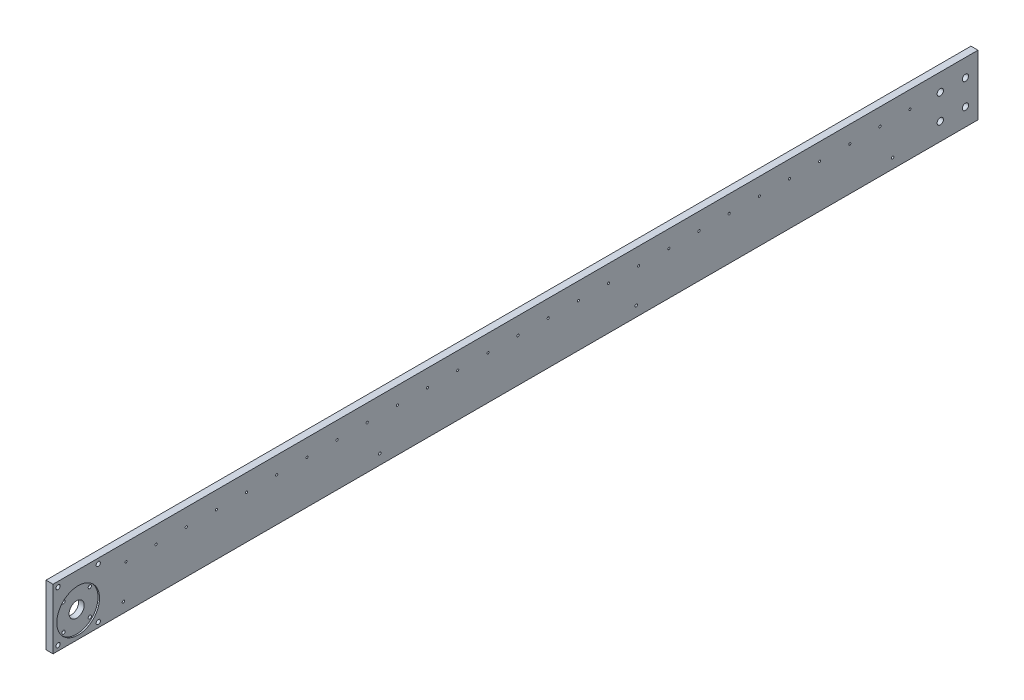
SolidWorks part; units mm, degrees
ref_plane "前视基准面" through (0, 0, 0) normal (0, 0, 1) x (1, 0, 0)
ref_plane "上视基准面" through (0, 0, 0) normal (0, 1, 0) x (1, 0, 0)
ref_plane "右视基准面" through (0, 0, 0) normal (1, 0, 0) x (0, 0, -1)
sketch "草图1" plane through (0, 0, 0) normal (1, 0, 0) x (0, 0, -1)
  line L1 (-920, 60) -> (920, 60)
  line L2 (-920, 60) -> (-920, -60)
  line L3 (-920, -60) -> (920, -60)
  line L4 (920, 60) -> (920, -60)
  line L5 (-920, 60) -> (920, -60) construction
  line L6 (-920, -60) -> (920, 60) construction
  point P0 (0, 0)
  dimension "D1" = 1840
  dimension "D2" = 120
extrude "凸台-拉伸1" add sketch "草图1" along normal blind 14
hole_wizard "打孔尺寸(%根据)内六角圆柱头螺钉的类型1" positions "草图2" profile "草图3" counterbore size "M6" standard "GB" end condition through all
sketch "草图2" plane through (0, 0, 0) normal (1, 0, 0) x (0, 0, -1)
  line L0 (-860, -10) -> (-727.1684, -10) construction
  line L4 (920, 60) -> (-920, 60) construction
  line L5 (-843.837, 16.163) -> (-896.163, 16.163) construction
  line L7 (-843.837, 16.163) -> (-843.837, -36.163) construction
  line L9 (-870, 16.163) -> (-870, -28.2194) construction
  line L11 (-843.837, -10) -> (-896.4633, -10) construction
  line L13 (-843.837, 16.163) -> (-870, -10) construction
  line L14 (-920, 60) -> (-920, -60) construction
  point P0 (-896.163, 16.163)
  point P2 (-843.837, 16.163)
  point P4 (-896.163, -36.163)
  point P6 (-843.837, -36.163)
  dimension "D2" = 45
  dimension "D1" = 70
  dimension "D3" = 37
  dimension "D4" = 50
sketch "草图3" plane through (0, 16.163, 896.163) normal (0, 1, 0) x (0, 0, 1)
  line L0 (0, 0) -> (0, 14)
  line L1 (0, 14) -> (3.3, 14)
  line L3 (3.3, 14) -> (3.3, 6.8)
  line L4 (3.3, 6.8) -> (5.5, 6.8)
  line L5 (5.5, 6.8) -> (5.5, 0)
  line L7 (5.5, 0) -> (0, 0)
  line L11 (0, -6.35) -> (0, 107.95) construction
  dimension "通孔孔直径" = 6.6
  dimension "通孔孔深度" = 14
  dimension "柱形沉头孔直径" = 11
  dimension "柱形沉头孔深度" = 6.8
hole_wizard "M5 螺纹孔1" positions "草图4" profile "草图5" tap size "M5" standard "GB" end condition through all
sketch "草图4" plane through (14, 0, 0) normal (1, 0, 0) x (0, 0, -1)
  line L0 (-920, 60) -> (-920, -60) construction
  line L1 (-920, -60) -> (920, -60) construction
  point P0 (-775, 26)
  dimension "D1" = 145
  dimension "D2" = 86
sketch "草图5" plane through (14, 26, 775) normal (0, 1, 0) x (0, 0, -1)
  line L0 (0, 0) -> (0, 14)
  line L1 (0, 14) -> (2.1, 14)
  line L2 (2.1, 14) -> (2.1, 0)
  line L5 (2.1, 0) -> (0, 0)
  line L11 (0, -6.35) -> (0, 107.95) construction
  dimension "通孔螺纹孔钻头直径" = 4.2
  dimension "通孔螺纹孔钻头深度" = 14
cosmetic thread "孔螺蚊线1" parameters "D2"=5
pattern_linear "阵列(线性)1" count 27 spacing 60 along (0, 0, -1) of "M5 螺纹孔1"
hole_wizard "Ø12.5 (12.5) 直径孔2" positions "草图6" profile "草图7" hole size "Ø12.5" standard "GB" end condition through all
sketch "草图6" plane through (14, 0, 0) normal (1, 0, 0) x (0, 0, -1)
  line L0 (920, 0) -> (754.1821, 0) construction
  line L1 (920, -60) -> (920, 60) construction
  point P0 (845, 25)
  point P2 (895, 25)
  point P4 (845, -25)
  point P6 (895, -25)
  dimension "D1" = 50
  dimension "D2" = 25
  dimension "D3" = 50
sketch "草图7" plane through (14, 25, -845) normal (0, 1, 0) x (0, 0, -1)
  line L0 (0, 0) -> (0, 14)
  line L1 (0, 14) -> (6.25, 14)
  line L2 (6.25, 14) -> (6.25, 0)
  line L5 (6.25, 0) -> (0, 0)
  line L11 (0, -6.35) -> (0, 107.95) construction
  dimension "通孔孔直径" = 12.5
  dimension "通孔孔深度" = 14
sketch "草图8" plane through (14, 0, 0) normal (1, 0, 0) x (0, 0, -1)
  line L0 (-896.163, 16.163) -> (-843.837, -36.163) construction
  line L1 (-896.163, -36.163) -> (-843.837, 16.163) construction
  circle A1 centre (-870, -10) radius 15
  dimension "D1" = 30
extrude "切除-拉伸1" cut sketch "草图8" against normal through all
hole_wizard "M6 螺纹孔1" positions "草图9" profile "草图10" tap size "M6" standard "GB" end condition through all
sketch "草图9" plane through (0, 0, 0) normal (-1, 0, 0) x (0, 0, 1)
  line L0 (920, -60) -> (-920, -60) construction
  line L1 (920, 60) -> (920, -60) construction
  point P0 (780, -40)
  dimension "D1" = 20
  dimension "D2" = 140
sketch "草图10" plane through (0, -40, 780) normal (0, 1, 0) x (0, 0, 1)
  line L0 (0, 0) -> (0, 14)
  line L1 (0, 14) -> (2.5, 14)
  line L2 (2.5, 14) -> (2.5, 0)
  line L5 (2.5, 0) -> (0, 0)
  line L11 (0, -6.35) -> (0, 107.95) construction
  dimension "通孔螺纹孔钻头直径" = 5
  dimension "通孔螺纹孔钻头深度" = 14
cosmetic thread "孔螺蚊线2" parameters "D2"=6
pattern_linear "阵列(线性)2" count 4 spacing 510 along (0, 0, -1) of "M6 螺纹孔1"
hole_wizard "Ø8.5 (8.5) 直径孔1" positions "草图11" profile "草图12" hole size "Ø8.5" standard "GB" end condition through all
sketch "草图11" plane through (14, 0, 0) normal (1, 0, 0) x (0, 0, -1)
  line L0 (-920, 0) -> (-838.3961, 0) construction
  line L1 (-920, 60) -> (-920, -60) construction
  point P0 (-910, 50)
  point P2 (-830, 50)
  point P4 (-910, -50)
  point P6 (-830, -50)
  dimension "D1" = 10
  dimension "D2" = 80
  dimension "D3" = 100
sketch "草图12" plane through (14, 50, 910) normal (0, 1, 0) x (0, 0, -1)
  line L0 (0, 0) -> (0, 14)
  line L1 (0, 14) -> (4.25, 14)
  line L2 (4.25, 14) -> (4.25, 0)
  line L5 (4.25, 0) -> (0, 0)
  line L11 (0, -6.35) -> (0, 107.95) construction
  dimension "通孔孔直径" = 8.5
  dimension "通孔孔深度" = 14
sketch "草图13" plane through (14, 0, 0) normal (1, 0, 0) x (0, 0, -1)
  circle A0 centre (-870, -10) radius 42.5
  dimension "D1" = 85
extrude "切除-拉伸2" cut sketch "草图13" against normal blind 3
